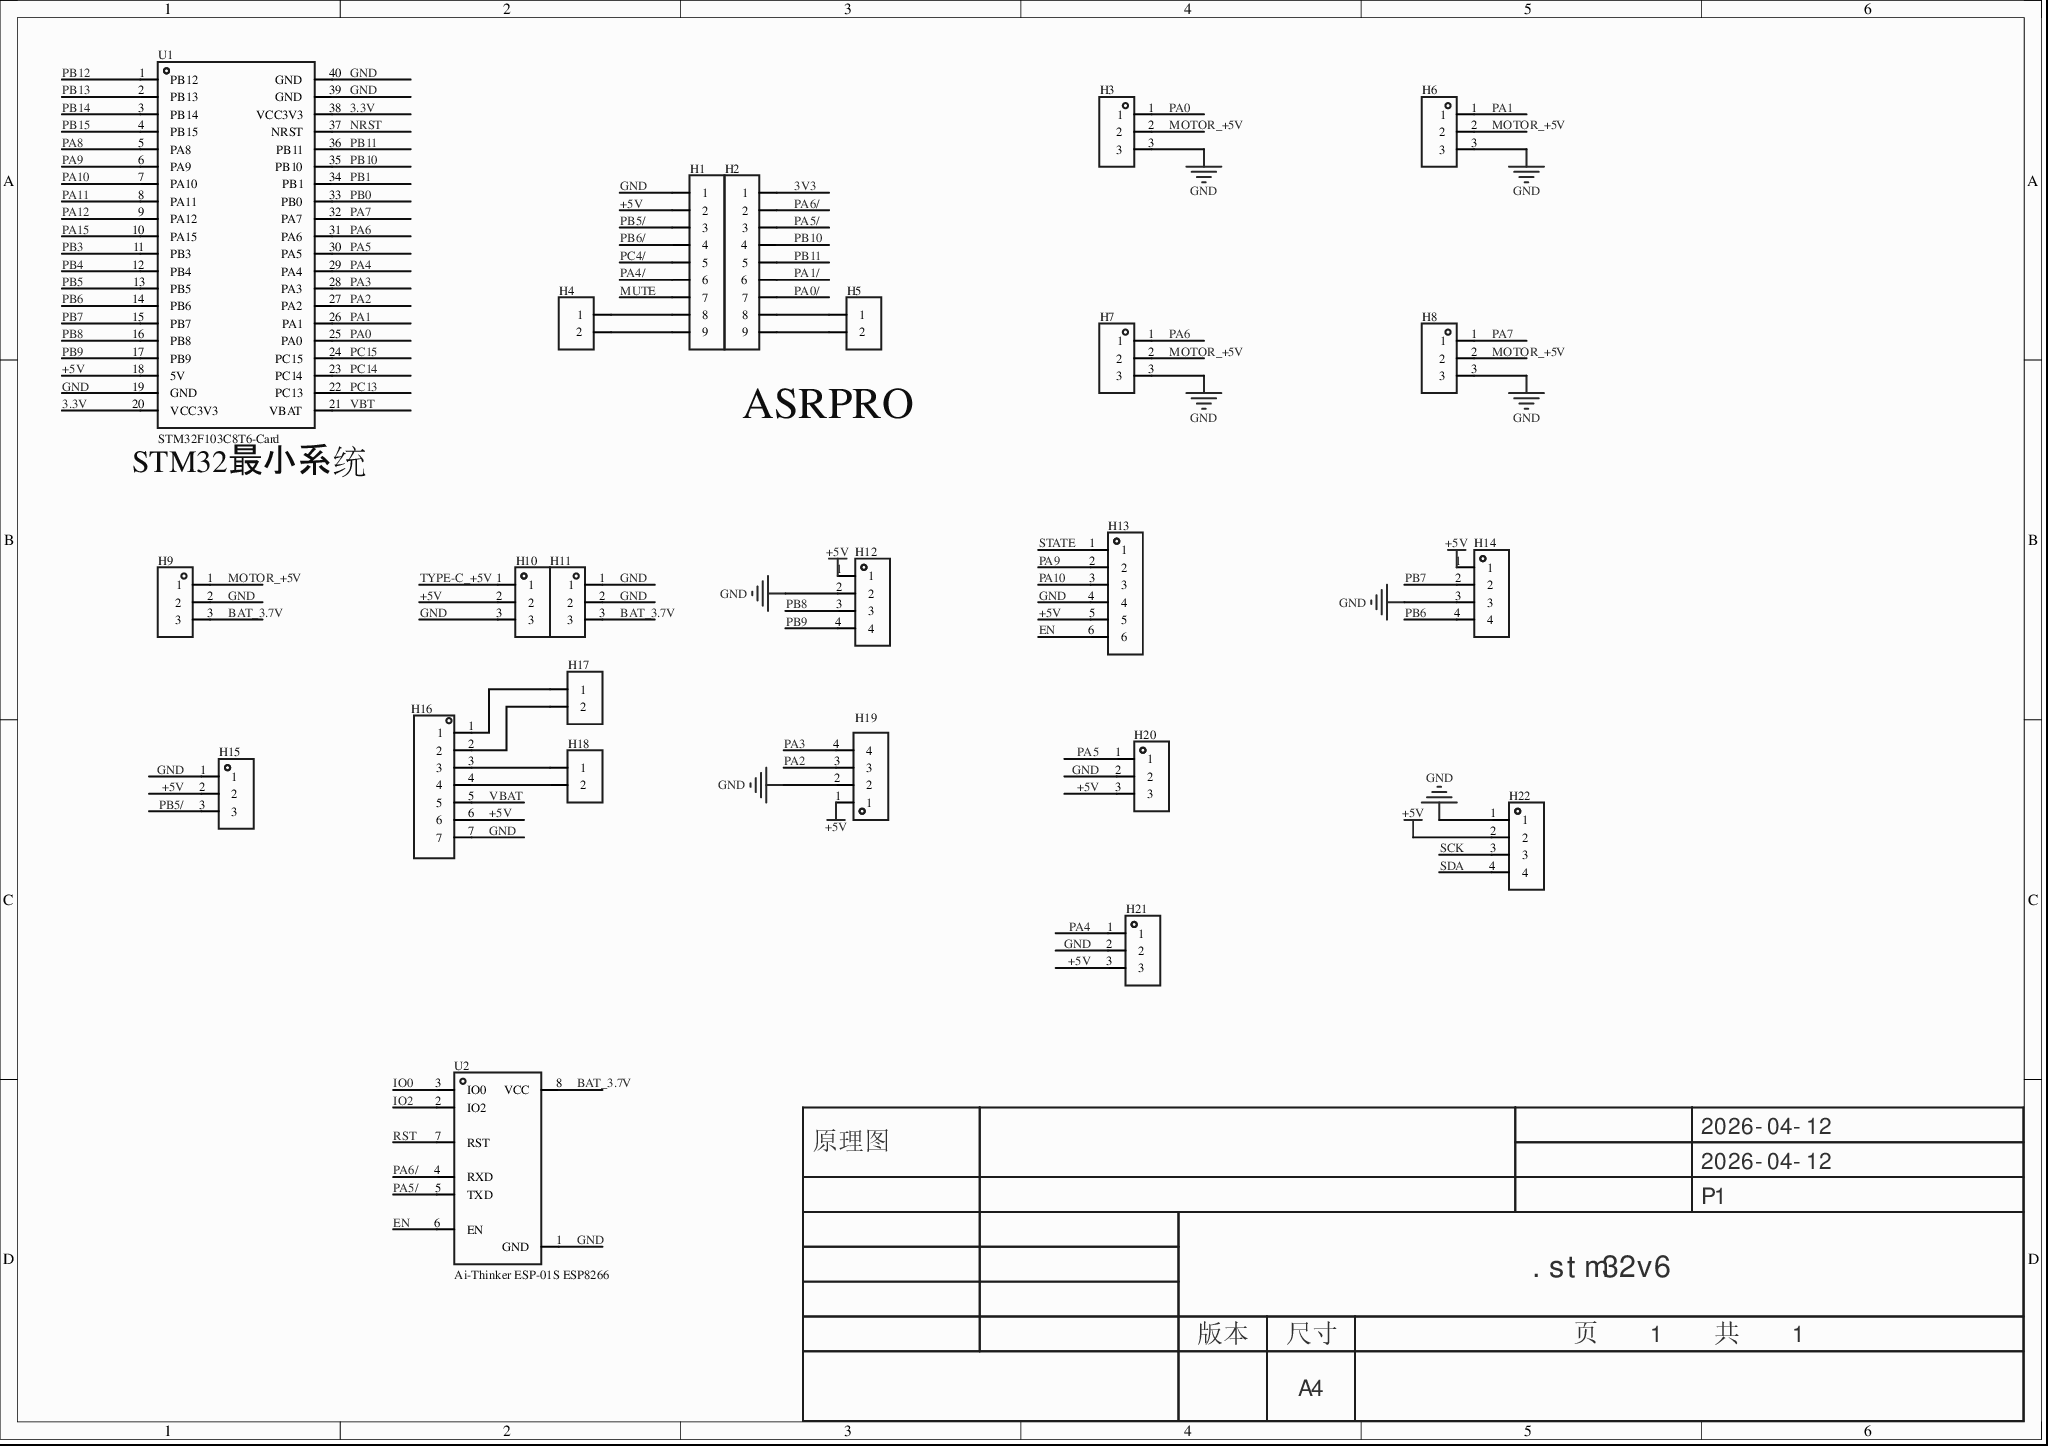
[diagram p0: MISC51489-3.schdoc]
# Altium project MISC51489-2.PrjPcb
1 sheet, 24 parts. Net scope: global (net labels, ports and power ports of the same name join across sheets).
Board file: MISC51489.pcbdoc

## Sheet MISC51489-3.schdoc
size 297 x 209 mm; Version: V1.0; @Project Name: MISC51489; @Page Count: 1; @Update Date: 2026-04-12; @Create Date: 2026-04-12; @Schematic Name: MISC51489; @Page No: 1; @Create Time: 23:22:16; @Update Time: 17:32:40; @Board Name: MISC51489

### Parts
H1  (no value)  [HDR-TH_9P-P2.54-V-F-1]
H2  (no value)  [HDR-TH_9P-P2.54-V-F-1]
H3  (no value)  [HDR-TH_3P-P2.54-V-F]
H4  (no value)  [HDR-TH_2P-P2.54-V-F]
H5  (no value)  [HDR-TH_2P-P2.54-V-F]
H6  (no value)  [HDR-TH_3P-P2.54-V-F]
H7  (no value)  [HDR-TH_3P-P2.54-V-F]
H8  (no value)  [HDR-TH_3P-P2.54-V-F]
H9  (no value)  [HDR-TH_3P-P2.54-V-F]
H10  (no value)  [HDR-TH_3P-P2.54-V-F]
H11  (no value)  [HDR-TH_3P-P2.54-V-F]
H12  (no value)  [HDR-TH_4P-P2.54-V-F]
H13  (no value)  [HDR-TH_6P-P2.54-V-F]
H14  (no value)  [HDR-TH_4P-P2.54-V-F]
H15  (no value)  [HDR-TH_3P-P2.54-V-F]
H16  (no value)  [HDR-TH_7P-P2.54-V-F]
H17  (no value)  [HDR-TH_2P-P2.54-V-F]
H18  (no value)  [HDR-TH_2P-P2.54-V-F]
H19  (no value)  [HDR-TH_4P-P2.54-V-F]
H20  (no value)  [HDR-TH_3P-P2.54-V-F]
H21  (no value)  [HDR-TH_3P-P2.54-V-F]
H22  (no value)  [HDR-TH_4P-P2.54-V-F]
U1  STM32F103C8T6-Card  [CONN-TH_L53.3-W22.9_STM32F103C8T6-CARD]
U2  Ai-Thinker ESP-01S ESP8266  [WIFIM-TH_8P-L24.7-W14.4-P2.54]

### Nets
+5V: H1.2 H10.2 H12.1 H13.5 H14.1 H15.2 H16.6 H19.1 H20.3 H21.3 H22.2 U1.18(5V)
GND: H1.1 H3.3 H6.3 H7.3 H8.3 H9.2 H10.3 H11.1 H11.2 H12.2 H13.4 H14.3 H15.1 H16.7 H19.2 H20.2 H21.2 H22.1 U1.19(GND) U1.39(GND) U1.40(GND) U2.1(GND)
3.3V: U1.20(VCC3V3) U1.38(VCC3V3)
3V3: H2.1
BAT_3.7V: H9.3 H11.3 U2.8(VCC)
EN: H13.6 U2.6(EN)
IO0: U2.3(IO0)
IO2: U2.2(IO2)
MOTOR_+5V: H3.2 H6.2 H7.2 H8.2 H9.1
MUTE: H1.7
NRST: U1.37(NRST)
PA0: H3.1 U1.25(PA0)
PA0/: H2.7
PA1: H6.1 U1.26(PA1)
PA1/: H2.6
PA2: H19.3 U1.27(PA2)
PA3: H19.4 U1.28(PA3)
PA4: H21.1 U1.29(PA4)
PA4/: H1.6
PA5: H20.1 U1.30(PA5)
PA5/: H2.3 U2.5(TXD)
PA6: H7.1 U1.31(PA6)
PA6/: H2.2 U2.4(RXD)
PA7: H8.1 U1.32(PA7)
PA8: U1.5(PA8)
PA9: H13.2 U1.6(PA9)
PA10: H13.3 U1.7(PA10)
PA11: U1.8(PA11)
PA12: U1.9(PA12)
PA15: U1.10(PA15)
PB0: U1.33(PB0)
PB1: U1.34(PB1)
PB3: U1.11(PB3)
PB4: U1.12(PB4)
PB5: U1.13(PB5)
PB5/: H1.3 H15.3
PB6: H14.4 U1.14(PB6)
PB6/: H1.4
PB7: H14.2 U1.15(PB7)
PB8: H12.3 U1.16(PB8)
PB9: H12.4 U1.17(PB9)
PB10: H2.4 U1.35(PB10)
PB11: H2.5 U1.36(PB11)
PB12: U1.1(PB12)
PB13: U1.2(PB13)
PB14: U1.3(PB14)
PB15: U1.4(PB15)
PC4/: H1.5
PC13: U1.22(PC13)
PC14: U1.23(PC14)
PC15: U1.24(PC15)
RST: U2.7(RST)
SCK: H22.3
SDA: H22.4
STATE: H13.1
TYPE-C_+5V: H10.1
VBAT: H16.5
VBT: U1.21(VBAT)
NetH1_8: H1.8 H4.1
NetH1_9: H1.9 H4.2
NetH2_8: H2.8 H5.1
NetH2_9: H2.9 H5.2
NetH16_1: H16.1 H17.1
NetH16_2: H16.2 H17.2
NetH16_3: H16.3 H18.1
NetH16_4: H16.4 H18.2

### Notes on the sheet
- ASRPRO
- (near U1) STM32最小系统
- 2026-04-12
- 原理图
- P1
- .stm32v6
- 版本
- 尺寸
- A4
- 页    1    共    1

### Library data of the parts
H1 H2 = HDR-F_2.54_1x9P: Symbol: Header-Female-2.54_1x9; AddInBom: yes; ModelId: 3a7016416d904017ac5ead6cc0f14e9c0819f05c4eef4c71ace90d822a990e87; ModelName: HDR-TH_9P-P2.54-F-LI-1X9P; ModelTransform: 915.746,94.488,0,0,0,0,0,0,-125.984; Device: HDR-F_2.54_1x9P; ConvertToPcb: yes; FootprintName: HDR-TH_9P-P2.54-V-F-1; SupplierPart: C39576; Supplier Footprint: 插件
H3 H6-H11 H15 H20 H21 = HDR-F_2.54_1x3P: Symbol: PM254V-11-03-H85; 3D Model: f3b3cc5aae9641bf9e56fc160cef875b; 3D Model Transform: 299.9994,100,0,0,0,0,0,0,-118.11; ConvertToPcb: yes; ModelName: HDR2.54-F-LI-1X3P; Device: HDR-F_2.54_1x3P; Supplier Part: C541850; Supplier Footprint: 插件; AddInBom: yes; FootprintName: HDR-TH_3P-P2.54-V-F
H4 H5 H17 H18 = HDR-F_2.54_1x2P: Symbol: Header-Female-2.54_1x2; ConvertToPcb: yes; ModelId: a9450ef445564560a104363b9aacde4e; ModelName: HDR-TH_2P-P2.54-F-LI-1X2P; ModelTransform: 215.7476,98.425,0,0,0,0,0,0,-129.921; Device: HDR-F_2.54_1x2P; AddInBom: yes; SupplierPart: C49661; Supplier Footprint: 插件; FootprintName: HDR-TH_2P-P2.54-V-F
H12 H14 H19 H22 = HDR-F_2.54_1x4P: Symbol: 2.54-1*4P母; ConvertToPcb: yes; ModelId: d187812051054f85879fcaa51a310d8e0819f05c4eef4c71ace90d822a990e87; ModelTransform: 419.6842,98.464,0,0,0,0,0,0,-118.11; Device: HDR-F_2.54_1x4P; AddInBom: yes; SupplierPart: C2718488; Supplier Footprint: 插件; FootprintName: HDR-TH_4P-P2.54-V-F; ModelName: HDR-TH_4P-P2.54-V-F
H13 = HDR-F_2.54_1x6P: Symbol: Header-Female-2.54_1x6; ConvertToPcb: yes; ModelId: 0f5bcf94dcda47d085f24cdca1696fe9; ModelTransform: 619.684,94.488,0,0,0,0,0,0,-125.984; Device: HDR-F_2.54_1x6P; AddInBom: yes; SupplierPart: C40877; Supplier Footprint: 插件; FootprintName: HDR-TH_6P-P2.54-V-F; ModelName: HDR-TH_6P-P2.54-V-F
H16 = HDR-F_2.54_1x7P: Symbol: 220S-1*7P H=8.5MM Ytype Gold-plated; ConvertToPcb: yes; ModelId: 4c31987253bc43b9b52c17be2a6d3f910819f05c4eef4c71ace90d822a990e87; ModelName: HDR-TH_7P-P2.54-F-LI-1X7P; ModelTransform: 715.7466,94.488,0,0,0,0,0,0,-118.11; Device: HDR-F_2.54_1x7P; AddInBom: yes; SupplierPart: C124418; Supplier Footprint: 插件; FootprintName: HDR-TH_7P-P2.54-V-F
U1 = STM32F103C8T6-Card: AddInBom: yes; Symbol: STM32F103C8T6-CARD; Device: STM32F103C8T6-Card; LCSC Part Name: STM32F103C8T6-Card; SupplierPart: C9900077949; ManufacturerPart: STM32F103C8T6-Card; Supplier Footprint: 插件; Supplier: LCSC; ConvertToPcb: yes; FootprintName: CONN-TH_L53.3-W22.9_STM32F103C8T6-CARD
U2 = Ai-Thinker ESP-01S ESP8266: Manufacturer: Ai-Thinker(安信可); AddInBom: yes; ModelId: 9453774c1eaa4779b246df5901e962460819f05c4eef4c71ace90d822a990e87; ModelName: WIFIM-TH_8P-L24.7-W14.4-H2.8-P2.54; ModelTransform: 972.43904,566.928,0,0,0,0,377.167,-3.936,-118.11; Symbol: AI-THINKER ESP-01S ESP8266; Device: Ai-Thinker ESP-01S ESP8266; LCSC Part Name: Ai-Thinker ESP-01S ESP8266; SupplierPart: C17606792; ManufacturerPart: Ai-Thinker ESP-01S ESP8266; Supplier Footprint: -; JLCPCB Part Class: Extended Part; Datasheet: https://item.szlcsc.com/datasheet/Ai-Thinker%2520ESP-01S%2520ESP8266/18736031.html; Supplier: LCSC; ConvertToPcb: yes; FootprintName: WIFIM-TH_8P-L24.7-W14.4-P2.54